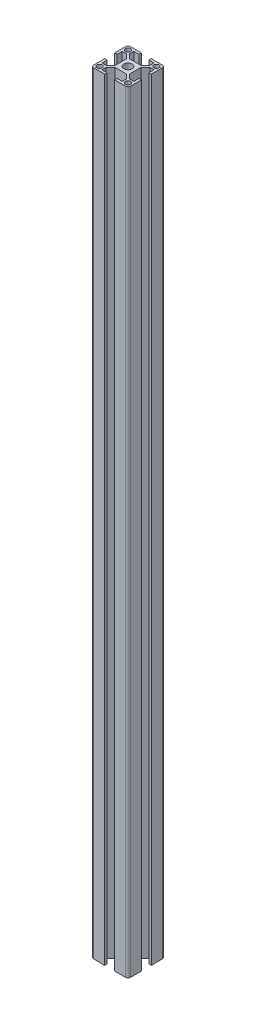
SolidWorks part; units mm, degrees
ref_plane "前视基准面" through (0, 0, 0) normal (0, 0, 1) x (1, 0, 0)
ref_plane "上视基准面" through (0, 0, 0) normal (0, 1, 0) x (1, 0, 0)
ref_plane "右视基准面" through (0, 0, 0) normal (1, 0, 0) x (0, 0, -1)
sketch "草图1" plane through (0, 0, 0) normal (0, 1, 0) x (1, 0, 0)
  line L44 (6.75, -28) -> (11, -28)
  line L45 (11, -28) -> (11, -30)
  line L46 (11, -30) -> (2, -30)
  line L47 (0, -28) -> (0, -19)
  line L48 (0, -19) -> (2, -19)
  line L49 (2, -19) -> (2, -23.25)
  line L50 (28, -30) -> (19, -30)
  line L51 (19, -30) -> (19, -28)
  line L52 (23.25, -28) -> (23.25, -24.6642)
  line L53 (19, -28) -> (23.25, -28)
  line L54 (30, -19) -> (30, -28)
  line L55 (28, -19) -> (30, -19)
  line L56 (28, -23.25) -> (28, -19)
  line L57 (24.6642, -23.25) -> (28, -23.25)
  line L58 (21, -19.5858) -> (24.6642, -23.25)
  line L59 (23.25, -24.6642) -> (19.5858, -21)
  line L60 (6.75, -24.6642) -> (6.75, -28)
  line L61 (2, -23.25) -> (5.3358, -23.25)
  line L62 (5.3358, -23.25) -> (9, -19.5858)
  line L63 (10.4142, -21) -> (6.75, -24.6642)
  line L64 (19.5858, -21) -> (10.4142, -21)
  line L65 (9, -19.5858) -> (9, -10.4142)
  line L66 (21, -10.4142) -> (21, -19.5858)
  line L67 (30, -11) -> (28, -11)
  line L68 (28, -11) -> (28, -6.75)
  line L69 (28, -6.75) -> (24.6642, -6.75)
  line L70 (24.6642, -6.75) -> (21, -10.4142)
  line L71 (19.5858, -9) -> (23.25, -5.3358)
  line L72 (10.4142, -9) -> (19.5858, -9)
  line L73 (6.75, -5.3358) -> (10.4142, -9)
  line L74 (9, -10.4142) -> (5.3358, -6.75)
  line L75 (2, -11) -> (0, -11)
  line L76 (2, -6.75) -> (2, -11)
  line L77 (5.3358, -6.75) -> (2, -6.75)
  line L78 (6.75, -2) -> (6.75, -5.3358)
  line L79 (23.25, -5.3358) -> (23.25, -2)
  line L80 (23.25, -2) -> (19, -2)
  line L81 (19, -2) -> (19, 0)
  line L82 (11, 0) -> (11, -2)
  line L83 (11, -2) -> (6.75, -2)
  line L84 (30, -2) -> (30, -11)
  line L85 (19, 0) -> (28, 0)
  line L86 (2, 0) -> (11, 0)
  line L87 (0, -11) -> (0, -2)
  line L88 (0, -15) -> (30, -15) construction
  line L89 (15, -30) -> (15, 0) construction
  line L90 (0, 0) -> (30, -30) construction
  line L91 (0, -30) -> (30, 0) construction
  arc A9 (0, -28) -> (2, -30) centre (2, -28) ccw
  circle A10 centre (3.375, -26.625) radius 2.1
  circle A11 centre (26.625, -26.625) radius 2.1
  arc A12 (28, -30) -> (30, -28) centre (28, -28) ccw
  circle A13 centre (15, -15) radius 3.4
  circle A14 centre (3.375, -3.375) radius 2.1
  circle A15 centre (26.625, -3.375) radius 2.1
  arc A16 (30, -2) -> (28, 0) centre (28, -2) ccw
  arc A17 (2, 0) -> (0, -2) centre (2, -2) ccw
  dimension "D2" = 15
  dimension "D5" = 6.8
  dimension "D8" = 6
  dimension "D11" = 23.25
  dimension "D12" = 3.375
  dimension "D13" = 23.25
  dimension "D14" = 4.2
  dimension "D15" = 2
  dimension "D16" = 2
  dimension "D23" = 2
  dimension "D24" = 2
  dimension "D1" = 15
  dimension "D3" = 45
  dimension "D4" = 45
  dimension "D6" = 30
  dimension "D7" = 30
  dimension "D9" = 12
  dimension "D10" = 3.375
  dimension "D17" = 11
  dimension "D18" = 8
  dimension "D19" = 2
  dimension "D20" = 2
  dimension "D21" = 11
  dimension "D22" = 8
  dimension "D25" = 2
  dimension "D26" = 2
  dimension "D27" = 6.75
  dimension "D28" = 16.5
  dimension "D29" = 6.75
  dimension "D30" = 16.5
  dimension "D31" = 12
  dimension "D32" = 6
  dimension "D33" = 2
  dimension "D34" = 1
  dimension "D35" = 2
  dimension "D36" = 1
extrude "拉伸1" add sketch "草图1" along normal blind 630
